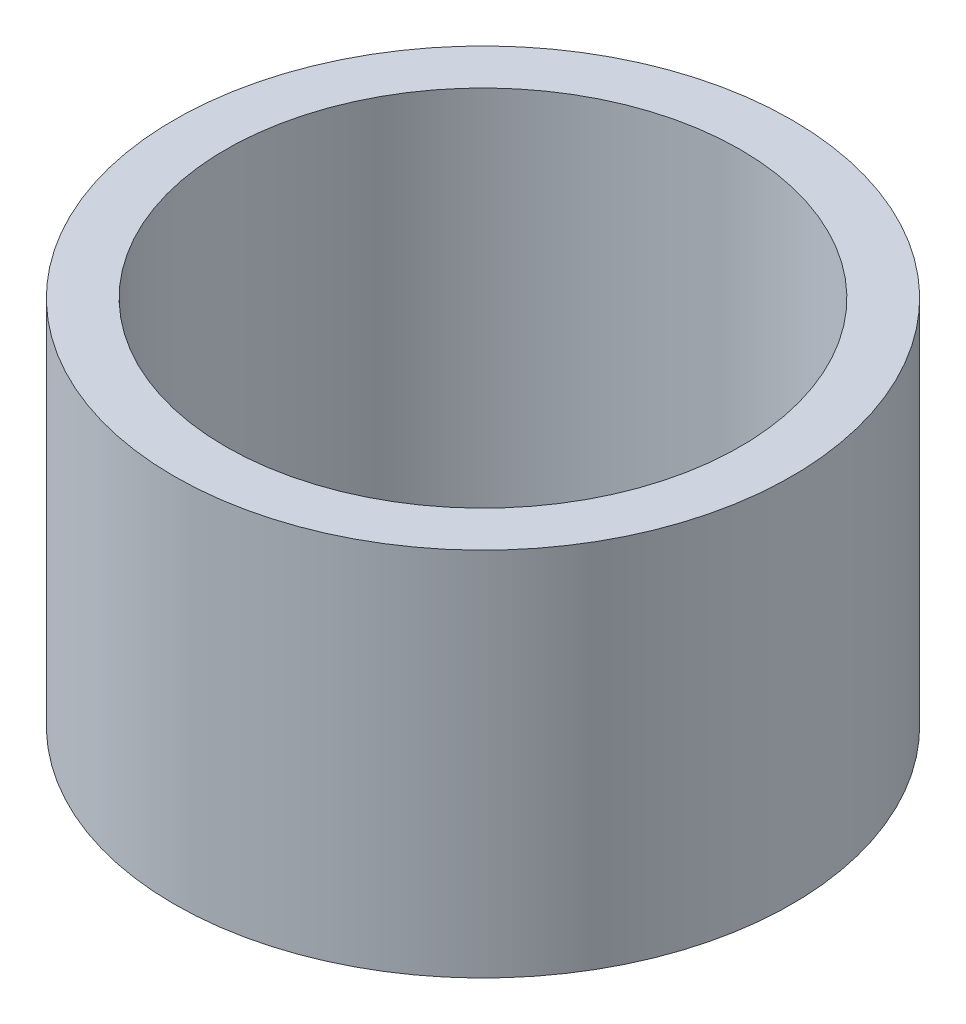
from build123d import *

# Parameters (mm, degrees)
SKETCH1_R           = 15
SKETCH1_R_2         = 12.5
BOSS_EXTRUDE1_DEPTH = 18


with BuildPart() as part:
    # Sketch1 → Boss-Extrude1 (new body)
    with BuildSketch(Plane(origin=(0, 0, 0), x_dir=(1, 0, 0), z_dir=(0, 1, 0))):
        with Locations(Location((0, 0, 0), (0, 0, 270))):
            Circle(SKETCH1_R)
        with Locations(Location((0, 0, 0), (0, 0, 270))):
            Circle(SKETCH1_R_2, mode=Mode.SUBTRACT)
    extrude(amount=BOSS_EXTRUDE1_DEPTH)


solid = part.part
